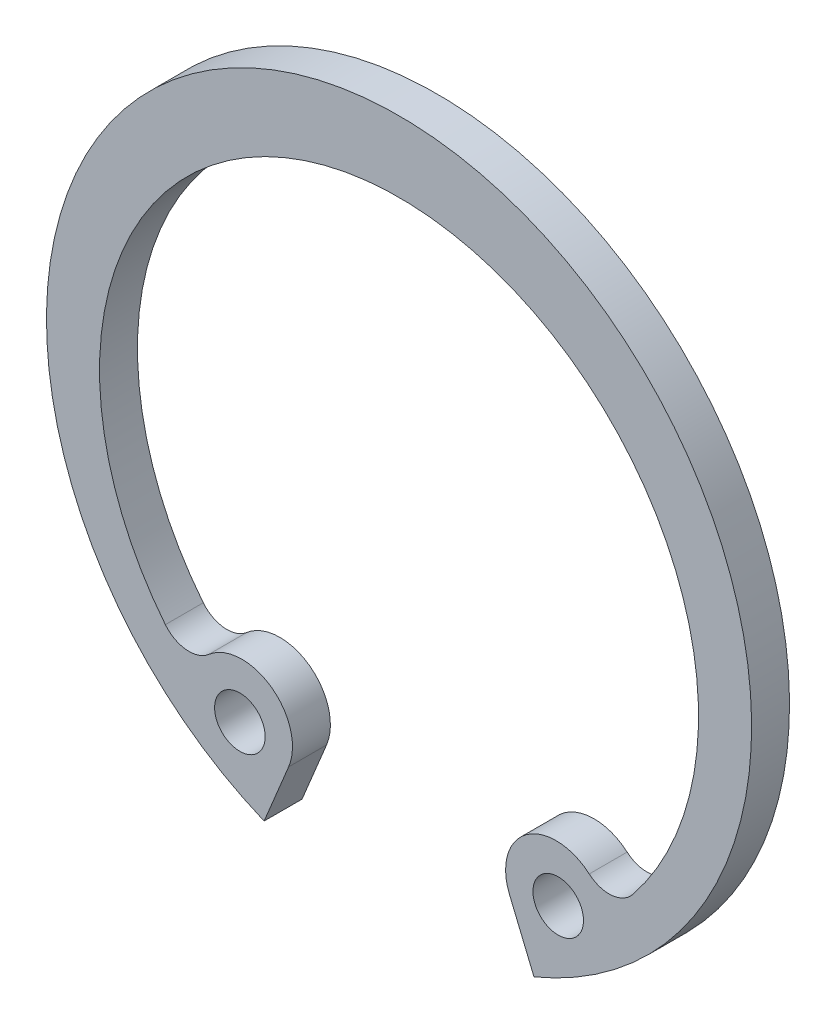
SolidWorks part; units mm, degrees
ref_plane "前视" through (0, 0, 0) normal (0, 0, 1) x (1, 0, 0)
ref_plane "上视" through (0, 0, 0) normal (0, 1, 0) x (1, 0, 0)
ref_plane "右视" through (0, 0, 0) normal (1, 0, 0) x (0, 0, -1)
sketch "尺寸草图" plane through (0, 0, 0) normal (0, 0, 1) x (1, 0, 0)
  line L0 (-13.95, 0) -> (13.95, 0) construction
  line L1 (0, 0) -> (-12.0811, -6.975) construction
  circle A0 centre (0, 0) radius 13.95
  point P5 (-9.75, 0)
  point P6 (10.6, 0)
  point P7 (2, 0)
  point P8 (11.8, 0)
  point P10 (-2.36, 0)
  point P11 (-0.7, 0)
  point P12 (-4.36, 0)
  point P13 (-10.95, 0)
  point P14 (26.8901, 15.525)
sketch "草图1" plane through (0, 0, 0) normal (0, 0, 1) x (1, 0, 0)
  line L0 (0, 13.95) -> (0, -12.8881) construction
  line L1 (-4.3688, -10.5471) -> (-5.3384, -12.8881)
  line L2 (-6.3797, -10.1756) -> (-6.2165, -9.7818) construction
  line L3 (0, 0) -> (-5.3384, -12.8881) construction
  line L4 (4.3688, -10.5471) -> (5.3384, -12.8881)
  arc A0 (5.3384, -12.8881) -> (-5.3384, -12.8881) centre (0, 0) ccw
  arc A1 (9.2459, -8.1118) -> (-9.2459, -8.1118) centre (0, -0.7) ccw
  circle A2 centre (-6.2981, -9.9787) radius 1
  arc A3 (-4.3688, -10.5471) -> (-7.5247, -8.2689) centre (-6.2165, -9.7818) ccw
  arc A4 (-7.5247, -8.2689) -> (-9.2459, -8.1118) centre (-8.3096, -7.3613) cw
  circle A5 centre (6.2981, -9.9787) radius 1
  arc A6 (4.3688, -10.5471) -> (7.5247, -8.2689) centre (6.2165, -9.7818) cw
  arc A7 (7.5247, -8.2689) -> (9.2459, -8.1118) centre (8.3096, -7.3613) ccw
extrude "基体-拉伸" add sketch "草图1" along normal blind 1.5
equation "\"D1@草图1\" = \"DD@尺寸草图\" "
equation "\"D2@草图1\"=\"d@尺寸草图\""
equation "\"D3@草图1\" = \"c@尺寸草图\""
equation "\"D6@草图1\" = \"RR@尺寸草图\""
equation "\"D8@草图1\" = \"R2@尺寸草图\""
equation "\"D7@草图1\" = \"R1@尺寸草图\""
equation "\"D4@草图1\" = \"aa@尺寸草图\"/2"
equation "\"D9@草图1\" = \"a@尺寸草图\""
equation "\"D5@草图1\" = \"d1@尺寸草图\""
equation "\"D1@基体-拉伸\" = \"s@尺寸草图\"/2"
equation "\"D2@基体-拉伸\" = \"D1@基体-拉伸\""
